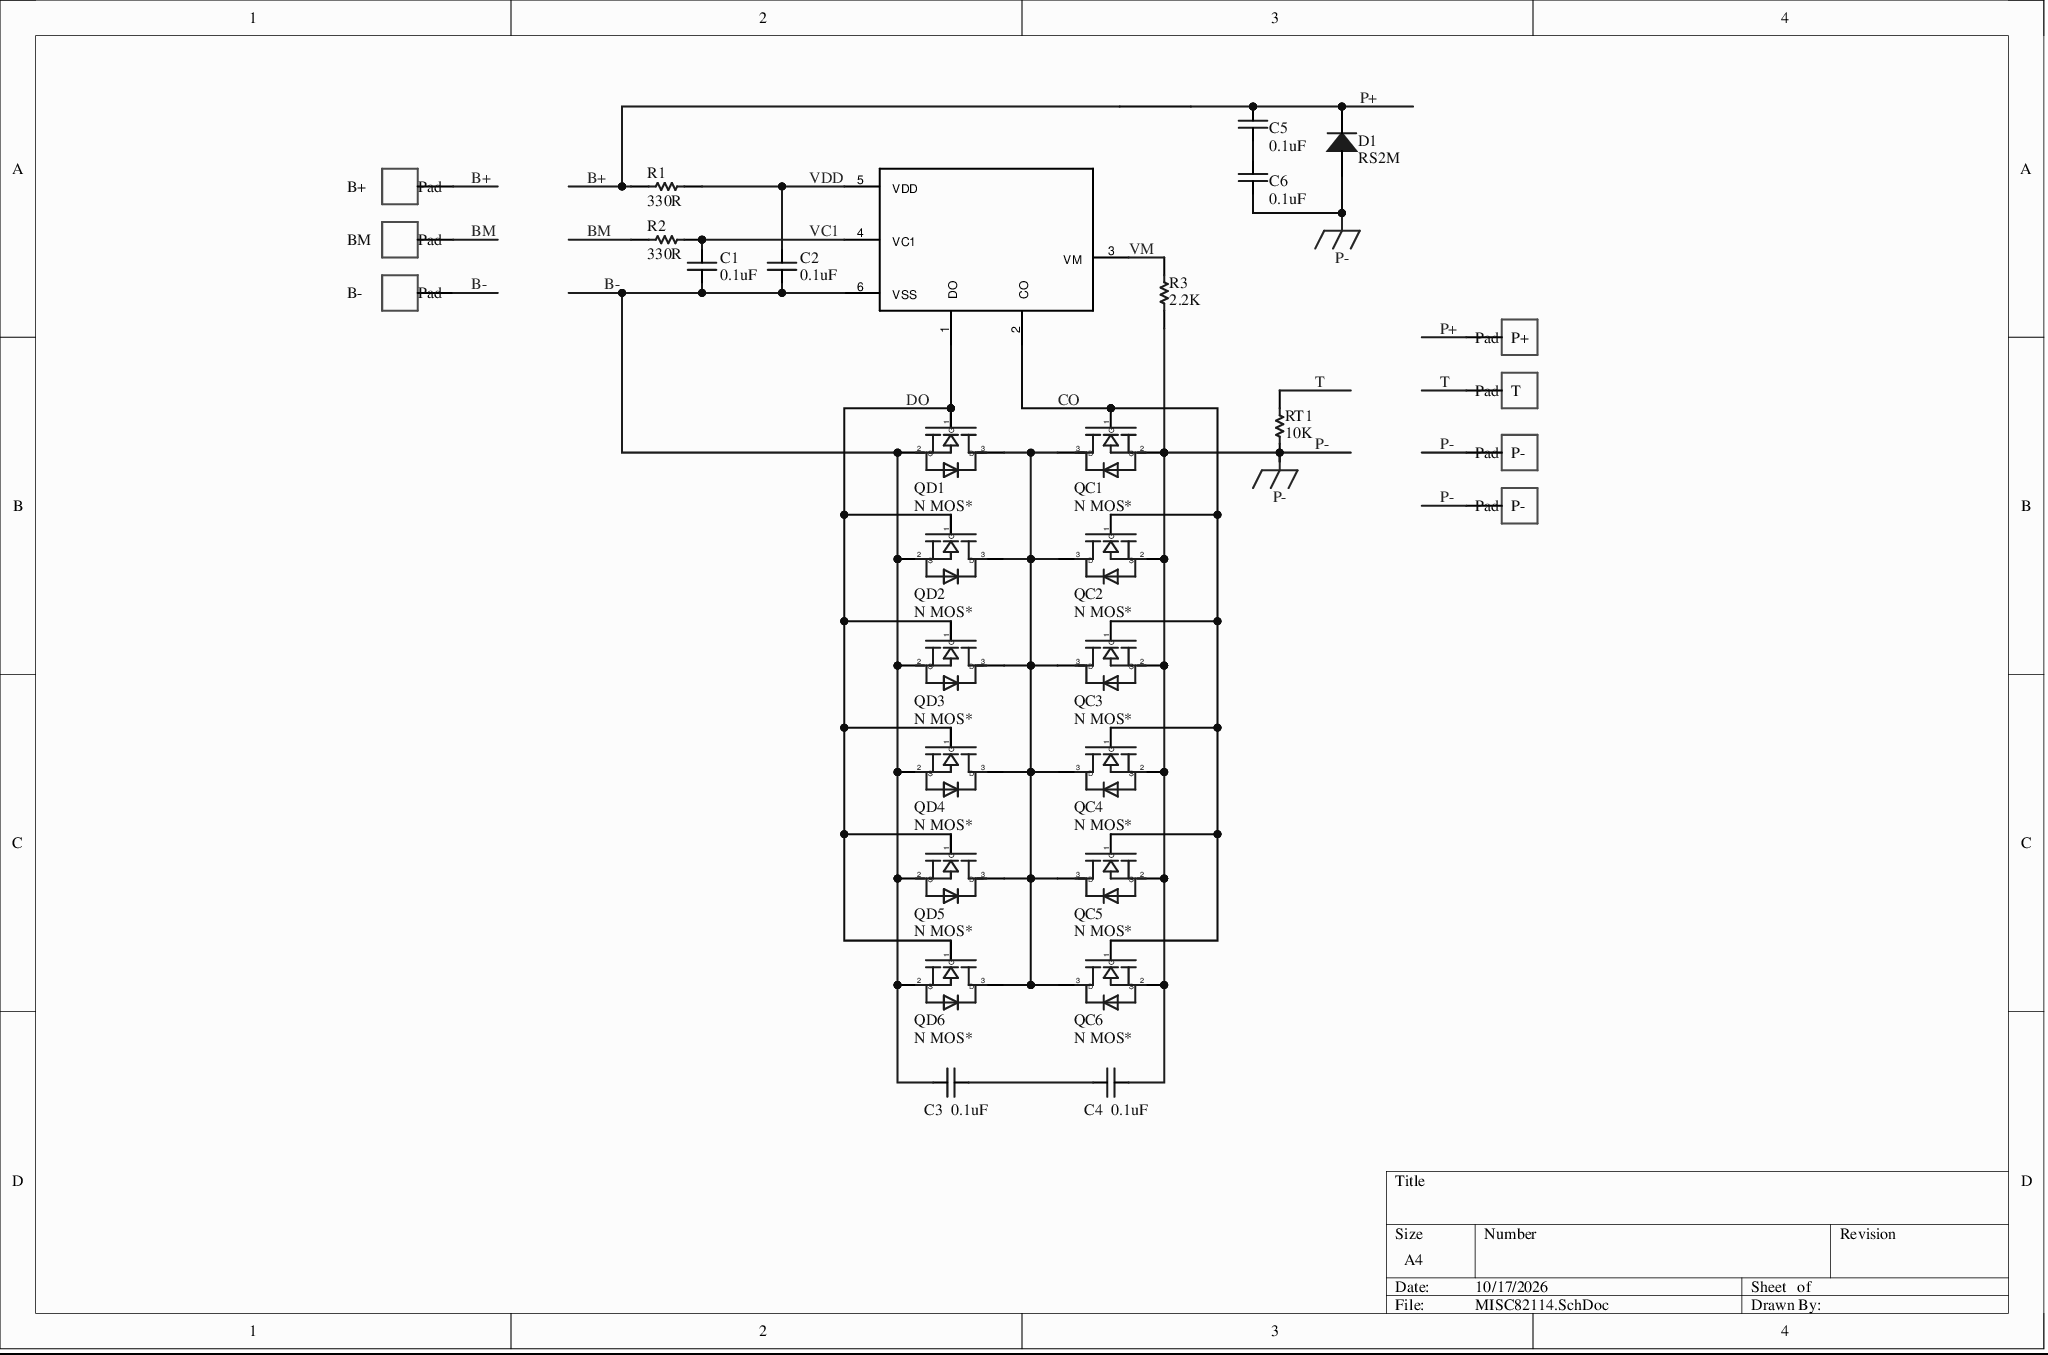
[diagram p0: MISC82114.SchDoc]
# Altium project MISC82114.PrjPcb
1 sheet, 31 parts. Net scope: global (net labels, ports and power ports of the same name join across sheets).
Board file: MISC82114.PcbDoc

## Sheet MISC82114.SchDoc
size A4; SheetNumber: 1; SheetTotal: 1

### Parts
(Parts that share a designator on the sheet are numbered #1, #2 ... from top to bottom, then left to right.)
B+  Pad  [Pad10X8mm]
B-  Pad  [Pad10X8mm]
BM  Pad  [Pad10X8mm]
C1  0.1uF  [C0603A]
C2  0.1uF  [C0603A]
C3  0.1uF  [C0603A]
C4  0.1uF  [C0603A]
C5  0.1uF  [C0603A]
C6  0.1uF  [C0603A]
D1  RS2M  [SMA(DO-214AC)]
P+  Pad  [Pad10X8mm]
P-#1  Pad  [Pad10X8mm]
P-#2  Pad  [Pad10X8mm]
QC1  N MOS*  [DFN-3x3L8(T3P)]
QC2  N MOS*  [DFN-3x3L8(T3P)]
QC3  N MOS*  [DFN-3x3L8(T3P)]
QC4  N MOS*  [DFN-3x3L8(T3P)]
QC5  N MOS*  [DFN-3x3L8(T3P)]
QC6  N MOS*  [DFN-3x3L8(T3P)]
QD1  N MOS*  [DFN-3x3L8(T3P)]
QD2  N MOS*  [DFN-3x3L8(T3P)]
QD3  N MOS*  [DFN-3x3L8(T3P)]
QD4  N MOS*  [DFN-3x3L8(T3P)]
QD5  N MOS*  [DFN-3x3L8(T3P)]
QD6  N MOS*  [DFN-3x3L8(T3P)]
R1  330R  [R0603A]
R2  330R  [R0603A]
R3  2.2K  [R0603A]
RT1  10K  [R0603A]
T  Pad  [Pad10X8mm]
U1  CW1025*  [SOT23-6A]  (value not drawn)

### Nets
P-: C4.1 C6.2 D1.2(K) P-#1.1 P-#2.1 QC1.2(S) QC2.2(S) QC3.2(S) QC4.2(S) QC5.2(S) QC6.2(S) R3.1 RT1.1
B+: B+.1 C5.1 D1.1(A) P+.1 R1.1  [also labelled P+]
B-: B-.1 C1.1 C2.1 C3.2 QD1.2(S) QD2.2(S) QD3.2(S) QD4.2(S) QD5.2(S) QD6.2(S) U1.6(VSS)
BM: BM.1 R2.1
CO: QC1.1(G) QC2.1(G) QC3.1(G) QC4.1(G) QC5.1(G) QC6.1(G) U1.2(CO)
DO: QD1.1(G) QD2.1(G) QD3.1(G) QD4.1(G) QD5.1(G) QD6.1(G) U1.1(DO)
T: RT1.2 T.1
VC1: C1.2 R2.2 U1.4(VC1)
VDD: C2.2 R1.2 U1.5(VDD)
VM: R3.2 U1.3(VM)
NetC3_1: C3.1 C4.2
NetC5_2: C5.2 C6.1
NetQC1_3: QC1.3(D) QC2.3(D) QC3.3(D) QC4.3(D) QC5.3(D) QC6.3(D) QD1.3(D) QD2.3(D) QD3.3(D) QD4.3(D) QD5.3(D) QD6.3(D)

### Library data of the parts
B+ B- BM P+ P-#1 P-#2 T = Pad: Connection pad (non-through-hole)
C1-C6 = CAP: SMD capacitor
D1 = RS2M: SMD diode
QC1-QC6 QD1-QD6 = N MOS*: SMD MOSFET
R1-R3 RT1 = RES: SMD resistor
U1 = CW1025*: 1-2S battery protection IC; Symbol: CW1025; Add into BOM: yes; Device: CW1025; Convert to PCB: yes